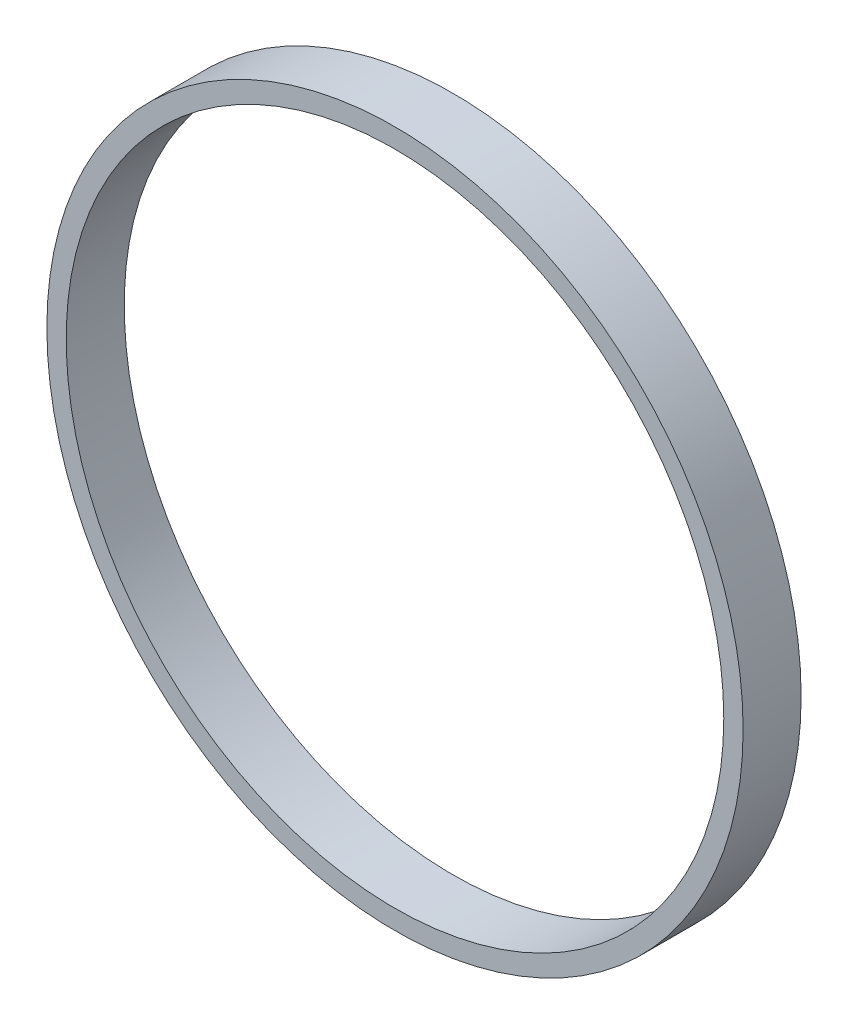
SolidWorks part; units mm, degrees
ref_plane "Front Plane" through (0, 0, 0) normal (0, 0, 1) x (1, 0, 0)
ref_plane "Top Plane" through (0, 0, 0) normal (0, 1, 0) x (1, 0, 0)
ref_plane "Right Plane" through (0, 0, 0) normal (1, 0, 0) x (0, 0, -1)
other "Configuration Table"
sketch "Sketch2" plane through (0, 0, 0) normal (0, 0, 1) x (1, 0, 0)
  circle A0 centre (0, 0) radius 90
  circle A1 centre (0, 0) radius 85
  dimension "D1" = 180
  dimension "D2" = 170
extrude "Boss-Extrude1" add sketch "Sketch2" along normal blind 15
